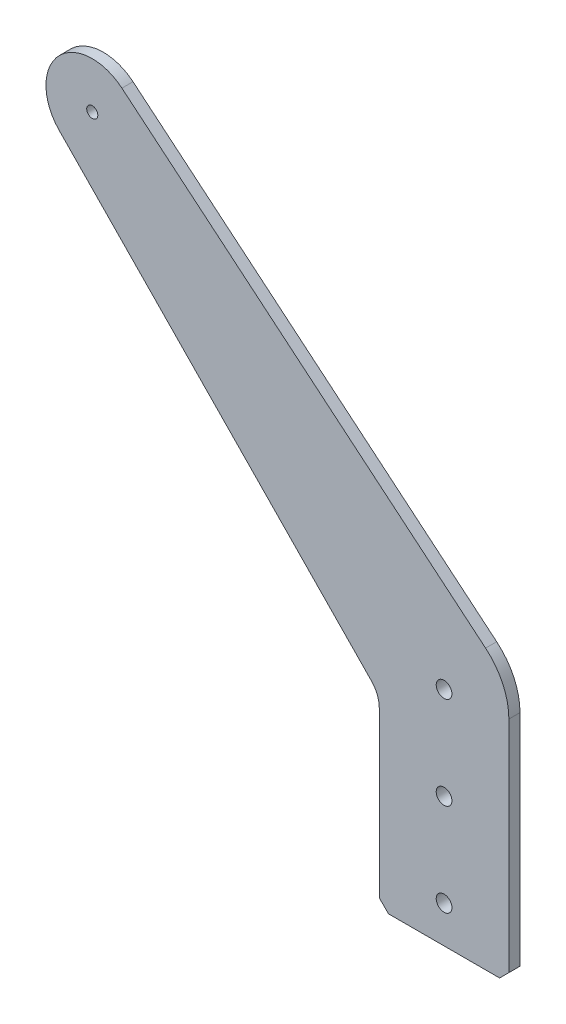
SolidWorks part; units mm, degrees
material "1023 碳钢板 (SS)"
ref_plane "前视基准面" through (0, 0, 0) normal (0, 0, 1) x (1, 0, 0)
ref_plane "上视基准面" through (0, 0, 0) normal (0, 1, 0) x (1, 0, 0)
ref_plane "右视基准面" through (0, 0, 0) normal (1, 0, 0) x (0, 0, -1)
sketch "草图1" plane through (0, 0, 0) normal (0, 0, 1) x (1, 0, 0)
  line L0 (16.0069, 19.2036) -> (212.4097, -144.5055)
  line L1 (225, -171.3906) -> (225, -295)
  line L2 (225, -295) -> (155, -295)
  line L3 (155, -295) -> (155, -201.097)
  line L4 (150.7463, -190.632) -> (-17.9105, -17.4417)
  arc A0 (16.0069, 19.2036) -> (-17.9105, -17.4417) centre (0, 0) ccw
  circle A1 centre (0, 0) radius 3
  arc A2 (155, -201.097) -> (150.7463, -190.632) centre (140, -201.097) ccw
  arc A3 (212.4097, -144.5055) -> (225, -171.3906) centre (190, -171.3906) cw
  circle A4 centre (190, -275) radius 4.25
  circle A5 centre (190, -225) radius 4.25
  circle A6 centre (190, -175) radius 4.25
  point P11 (155, -195)
  point P14 (225, -155)
  dimension "D1" = 50
  dimension "D7" = 6
  dimension "D8" = 15
  dimension "D9" = 35
  dimension "D13" = 8.5
  dimension "D2" = 225
  dimension "D3" = 70
  dimension "D4" = 100
  dimension "D5" = 140
  dimension "D6" = 295
  dimension "D10" = 50
  dimension "D11" = 100
  dimension "D12" = 35
  dimension "D14" = 20
extrude "凸台-拉伸1" add sketch "草图1" along normal blind 6
chamfer "倒角1" distance 5 angle 45 2 edges at (225, -295, 3) (155, -295, 3)
